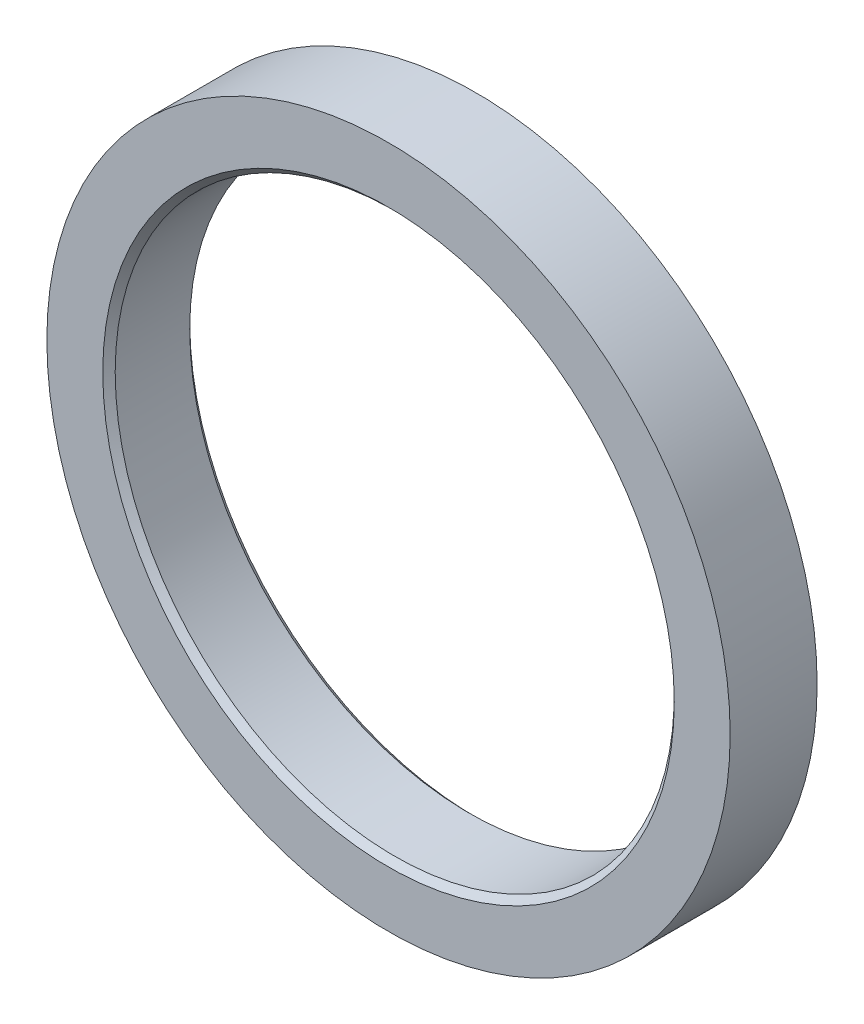
SolidWorks part; units mm, degrees
ref_plane "Front Plane" through (0, 0, 0) normal (0, 0, 1) x (1, 0, 0)
ref_plane "Top Plane" through (0, 0, 0) normal (0, 1, 0) x (1, 0, 0)
ref_plane "Right Plane" through (0, 0, 0) normal (1, 0, 0) x (0, 0, -1)
ref_plane "Plane1" through (0, 40.2756, 0) normal (0, -1, 0) x (1, 0, 0)
sketch "Sketch1" plane through (0, 40.2756, 0) normal (0, -1, 0) x (1, 0, 0)
  line L0 (475.7742, -188.193) -> (476.2742, -188.693)
  line L1 (476.2742, -188.693) -> (480.7742, -188.693)
  line L2 (480.7742, -188.693) -> (480.7742, -181.693)
  line L3 (480.7742, -181.693) -> (476.2742, -181.693)
  line L4 (476.2742, -181.693) -> (475.7742, -182.193)
  line L5 (475.7742, -182.193) -> (475.7742, -188.193)
  line L6 (453.2742, -181.693) -> (453.2742, -188.693) construction
  dimension "D1" = 22.5
  dimension "D2" = 23
  dimension "D3" = 27.5
  dimension "D4" = 0.5
  dimension "D5" = 6.5
  dimension "D6" = 7
revolve "Revolve1" add sketch "Sketch1" angle 360 about L6
